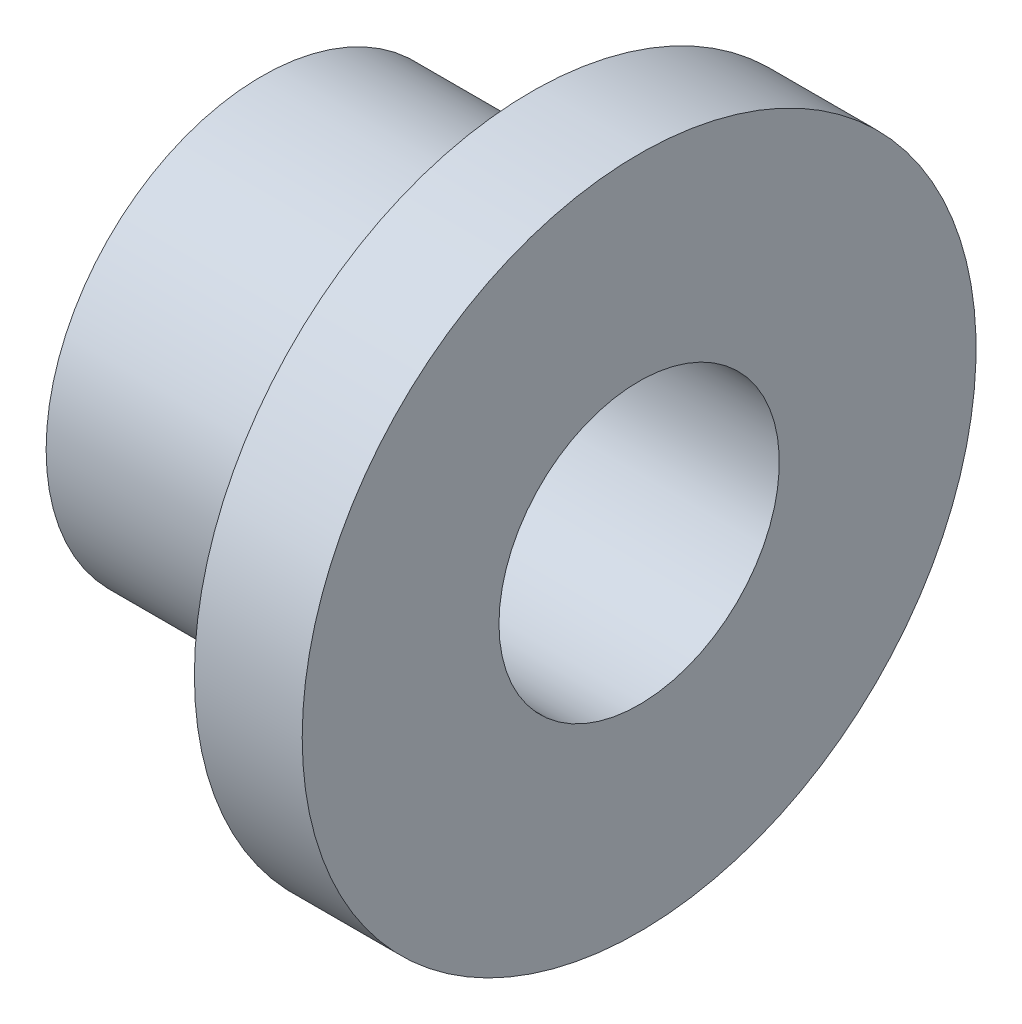
SolidWorks part; units mm, degrees
material "35"
ref_plane "Front Plane" through (0, 0, 0) normal (0, 0, 1) x (1, 0, 0)
ref_plane "Top Plane" through (0, 0, 0) normal (0, 1, 0) x (1, 0, 0)
ref_plane "Right Plane" through (0, 0, 0) normal (1, 0, 0) x (0, 0, -1)
sketch "Sketch1" plane through (0, 0, 0) normal (0, 0, 1) x (1, 0, 0)
  line L0 (0, 0) -> (78.9231, 0) construction
  line L1 (0, -26) -> (0, -40)
  line L2 (0, -40) -> (50, -40)
  line L3 (50, -40) -> (50, -62.5)
  line L4 (50, -62.5) -> (70, -62.5)
  line L5 (70, -62.5) -> (70, -26)
  line L6 (70, -26) -> (0, -26)
  dimension "D1" = 26
  dimension "D2" = 40
  dimension "D3" = 62.5
  dimension "D4" = 70
  dimension "D5" = 50
revolve "Revolve1" add sketch "Sketch1" angle 360 about L0
cosmetic thread "Cosmetic Thread1" parameters "D2"=60
